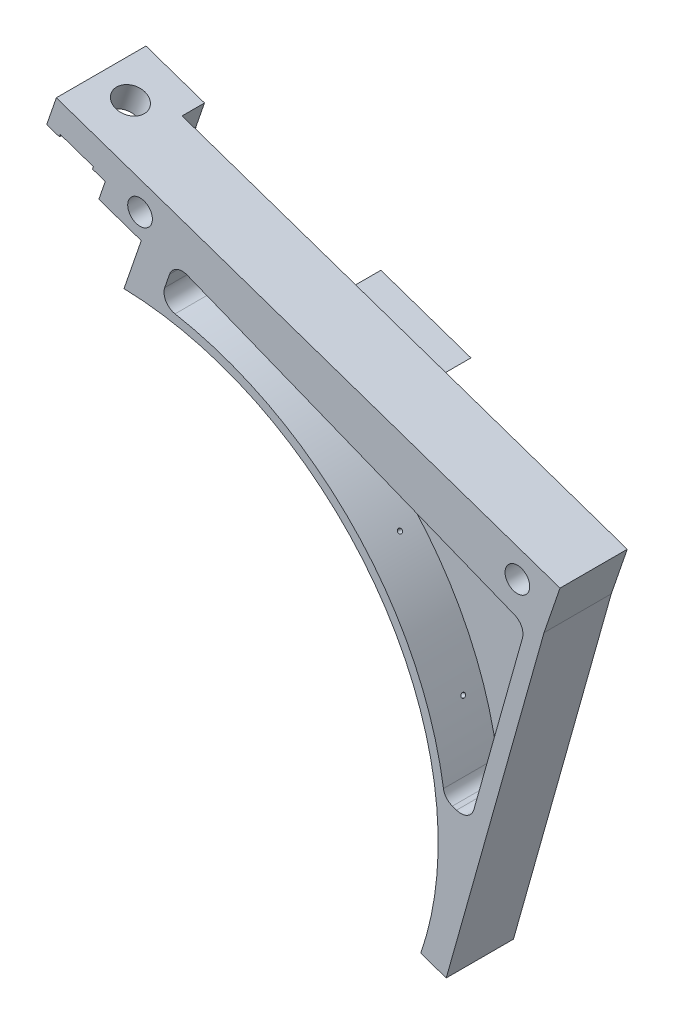
from build123d import *

# Parameters (mm, degrees)
EXTRUDE_1_DEPTH     = 8
SKETCH_2_R          = 2.75
EXTRUDE_2_DEPTH     = 15
CUT_EXTRUDE_1_DEPTH = 15
CUT_EXTRUDE_2_DEPTH = 8
CUT_EXTRUDE_3_DEPTH = 317.803371085
SKETCH_7_R          = 0.5
CUT_EXTRUDE_4_DEPTH = 311.990149374
EXTRUDE_3_DEPTH     = 15
SKETCH_9_W          = 10.8
SKETCH_9_H          = 20
EXTRUDE_4_DEPTH     = 6
EXTRUDE_5_REACH     = 320.172
SKETCH_12_W         = 3.25
SKETCH_12_H         = 42.464469098
EXTRUDE_6_DEPTH     = 15
CUT_EXTRUDE_5_DEPTH = 12
HOLE_WIZARD_M3_1_D  = 2.5


with BuildPart() as part:
    # 草图1 → 凸台-拉伸1 (new body)
    with BuildSketch(Plane.XY):
        Polygon((-181.873786677, 171.373096295), (-174.908927271, 177.441379972), (-194.997272817, 184.33298428), (-193.224414699, 175.267097261), align=None)
    extrude(amount=-EXTRUDE_1_DEPTH)



with BuildPart() as body_2:
    # 草图2 → 凸台-拉伸2 (new body)
    with BuildSketch(Plane.XY):
        with BuildLine():
            Line((-234.92191194, 189.572040939), (-267.921572877, 171.97259121))
            ThreePointArc((-267.921572877, 171.97259121), (-290.600732502, 153.720356817), (-305.007767585, 128.423604423))
            Line((-305.007767585, 128.423604423), (-293.655216332, 124.535156375))
            ThreePointArc((-293.655216332, 124.535156375), (-209.829850624, 165.587660123), (-168.777346876, 81.762294415))
            Line((-168.777346876, 81.762294415), (-157.424795623, 77.873846368))
            Line((-157.424795623, 77.873846368), (-135.603916755, 155.499532484))
            Line((-135.603916755, 155.499532484), (-132.034415869, 165.904274837))
            Line((-132.034415869, 165.904274837), (-231.352411054, 199.976783292))
            Line((-231.352411054, 199.976783292), (-234.92191194, 189.572040939))
        make_face()
        with Locations((-141.5485017, 162.824961471)):
            Circle(SKETCH_2_R, mode=Mode.SUBTRACT)
        with Locations((-225.73232619, 191.705468637)):
            Circle(SKETCH_2_R, mode=Mode.SUBTRACT)
        Polygon((-193.224414699, 175.267097261), (-181.873786677, 171.373096295), (-174.908927271, 177.441379972), (-194.997272817, 184.33298428), align=None, mode=Mode.SUBTRACT)
    extrude(amount=EXTRUDE_2_DEPTH)

    # 草图4 → 切除-拉伸1 (cut)
    with BuildSketch(Plane.XY.offset(15)):
        with BuildLine():
            Line((-207.885629626, 171.263926916), (-296.983281013, 201.781436227))
            Line((-296.983281013, 201.781436227), (-325.469194549, 118.615147397))
            Line((-325.469194549, 118.615147397), (-168.25634164, 64.766986109))
            Line((-168.25634164, 64.766986109), (-163.101080083, 79.818073417))
            ThreePointArc((-163.101080083, 79.818073417), (-166.554298483, 134.81618407), (-207.885629626, 171.263926916))
        make_face()
    extrude(amount=-CUT_EXTRUDE_1_DEPTH, mode=Mode.SUBTRACT)

    # 草图5 → 切除-拉伸2 (cut)
    with BuildSketch(Plane.XY.offset(15)):
        Polygon((-234.92191194, 189.572040939), (-225.463055256, 186.327040134), (-228.266951451, 178.153959799), (-237.725808135, 181.398960604), (-253.997826946, 186.981317532), (-251.193930751, 195.154397867), align=None)
    extrude(amount=-CUT_EXTRUDE_2_DEPTH, mode=Mode.SUBTRACT)

    # 草图6 → 切除-拉伸3 (cut, through all)
    with BuildSketch(Plane.XY.offset(7)):
        Polygon((-234.92191194, 189.572040939), (-237.695517736, 181.474336773), (-249.379698977, 185.476373912), (-246.606093182, 193.574078078), align=None)
    extrude(amount=-CUT_EXTRUDE_3_DEPTH, mode=Mode.SUBTRACT)

    # 草图7 → 切除-拉伸4 (cut, through all)
    with BuildSketch(Plane.XY.offset(7)):
        with Locations((-231.579880599, 183.90218604)):
            Circle(SKETCH_7_R)
    extrude(amount=-CUT_EXTRUDE_4_DEPTH, mode=Mode.SUBTRACT)

    # 草图8 → 凸台-拉伸3 (add)
    with BuildSketch(Plane.XY.offset(15)):
        with BuildLine():
            Line((-229.30663116, 175.123396184), (-228.239037464, 178.235326314))
            Line((-228.239037464, 178.235326314), (-207.885629626, 171.263926916))
            ThreePointArc((-207.885629626, 171.263926916), (-218.449445961, 174.007796146), (-229.30663116, 175.123396184))
        make_face()
    extrude(amount=-EXTRUDE_3_DEPTH)

    # 草图9 → 凸台-拉伸4 (add)
    with BuildSketch(Plane(origin=(35.072389683, 102.232550158, 0), x_dir=(0.9458856684293919, -0.324500080523692, 0), z_dir=(0.32450008052369195, 0.9458856684293918, 0))):
        with Locations((-289.125412254, -5)):
            Rectangle(SKETCH_9_W, SKETCH_9_H)
    extrude(amount=EXTRUDE_4_DEPTH)

    # 凸台-拉伸5: up to this face of the body (flat: up to its plane)
    extrude_5_end = Plane(body_2.part.faces().sort_by_distance((-237.433693905, 198.891426721, -5))[0])
    # 草图10 → 凸台-拉伸5 (add, up to the picked face)
    with BuildSketch(Plane.XY.offset(15), mode=Mode.PRIVATE) as extrude_5_sk1:
        Polygon((-236.331768591, 194.707438122), (-236.137068543, 195.274969523), (-233.255345678, 194.286351836), (-233.450045726, 193.718820435), align=None)
    extrude_5_tool1 = split(extrude(extrude_5_sk1.sketch, amount=-EXTRUDE_5_REACH, mode=Mode.PRIVATE), bisect_by=extrude_5_end, keep=Keep.BOTH, mode=Mode.PRIVATE)
    # 草图10 → 凸台-拉伸5 (add, up to the picked face)
    with BuildSketch(Plane.XY.offset(15), mode=Mode.PRIVATE) as extrude_5_sk2:
        Polygon((-243.709676805, 197.23853875), (-246.54733381, 198.212038991), (-244.405633279, 204.454884403), (-241.567976273, 203.481384162), align=None)
    extrude_5_tool2 = split(extrude(extrude_5_sk2.sketch, amount=-EXTRUDE_5_REACH, mode=Mode.PRIVATE), bisect_by=extrude_5_end, keep=Keep.BOTH, mode=Mode.PRIVATE)
    add(extrude_5_tool1.solids().sort_by(Axis((-234.793557, 194.496895, 15), (0, 0, -1)))[0])
    add(extrude_5_tool2.solids().sort_by(Axis((-244.057655, 200.846712, 15), (0, 0, -1)))[0])

    # 草图12 → Ø1.0 (1) 直径孔1 (revolve, cut)
    with BuildSketch(Plane(origin=(-239.82602265, 196.540519837, 5), x_dir=(0.9458856684293919, -0.32450008052369167, 0), z_dir=(0, 0, 1))):
        with Locations((1.625, 21.232234549)):
            Rectangle(SKETCH_12_W, SKETCH_12_H)
    revolve(axis=Axis((-241.886598161, 190.534145842, 5), (0.3245000805236916, 0.945885668429392, 0)), mode=Mode.SUBTRACT)


with BuildPart() as part_1:
    add(part.part)

    add(body_2.part)  # 凸台-拉伸6 merges body 2
    # 草图13 → 凸台-拉伸6 (add)
    with BuildSketch(Plane.XY):
        Polygon((-193.224414699, 175.267097261), (-181.873786677, 171.373096295), (-174.908927271, 177.441379972), (-194.997272817, 184.33298428), align=None)
    extrude(amount=EXTRUDE_6_DEPTH)

    # 草图14 → 切除-拉伸5 (cut)
    with BuildSketch(Plane.XY.offset(15)):
        with BuildLine():
            ThreePointArc((-156.047834036, 111.774217336), (-157.378743964, 112.691016779), (-158.04090319, 114.165258148))
            ThreePointArc((-158.04090319, 114.165258148), (-178.080420962, 154.651932226), (-217.922197627, 175.944792124))
            ThreePointArc((-217.922197627, 175.944792124), (-219.971910037, 177.379794621), (-220.220905282, 179.86948426))
            Line((-220.220905282, 179.86948426), (-219.156952171, 182.97080244))
            ThreePointArc((-219.156952171, 182.97080244), (-217.571105228, 184.723649859), (-215.208108923, 184.78392473))
            Line((-215.208108923, 184.78392473), (-142.189143758, 155.667074982))
            ThreePointArc((-142.189143758, 155.667074982), (-140.610396656, 154.208706418), (-140.412267192, 152.068606889))
            Line((-140.412267192, 152.068606889), (-151.259122885, 113.481956899))
            ThreePointArc((-151.259122885, 113.481956899), (-152.753497975, 111.637181572), (-155.120685935, 111.456145455))
            Line((-155.120685935, 111.456145455), (-156.047834036, 111.774217336))
        make_face()
    extrude(amount=-CUT_EXTRUDE_5_DEPTH, mode=Mode.SUBTRACT)

    # 草图15 → 切除-旋转1 (revolve, cut)
    with BuildSketch(Plane.XY.offset(7.5)):
        Polygon((-205.4487383, 166.676640825), (-201.772468541, 175.740203913), (-201.309131883, 175.552270037), (-204.985401642, 166.488706949), align=None)
    revolve(axis=Axis((-205.4487383, 166.676640825, 7.5), (0.375867752200837, 0.9266733150660432, 0)), mode=Mode.SUBTRACT)

    # 草图16 → 切除-旋转2 (revolve, cut)
    with BuildSketch(Plane.XY.offset(7.5)):
        Polygon((-177.87310191, 149.277238135), (-169.262777578, 156.723015795), (-168.935726472, 156.344812709), (-177.546050805, 148.899035049), align=None)
    revolve(axis=Axis((-177.87310191, 149.277238135, 7.5), (0.75640617255012, 0.6541022107653192, 0)), mode=Mode.SUBTRACT)

    # 草图17 → 切除-旋转3 (revolve, cut)
    with BuildSketch(Plane.XY.offset(7.5)):
        Polygon((-166.361705167, 125.109435071), (-154.938042437, 128.977654623), (-154.777679293, 128.504068663), (-166.201342023, 124.63584911), align=None)
    revolve(axis=Axis((-166.361705167, 125.109435071, 7.5), (0.9471719210759217, 0.3207262881731836, 0)), mode=Mode.SUBTRACT)

    # M3 螺纹孔1 (through all)
    with Locations(Plane.XY.offset(7)):
        with Locations((-231.579880599, 183.90218604)):
            Hole(HOLE_WIZARD_M3_1_D / 2)


solid = part_1.part
